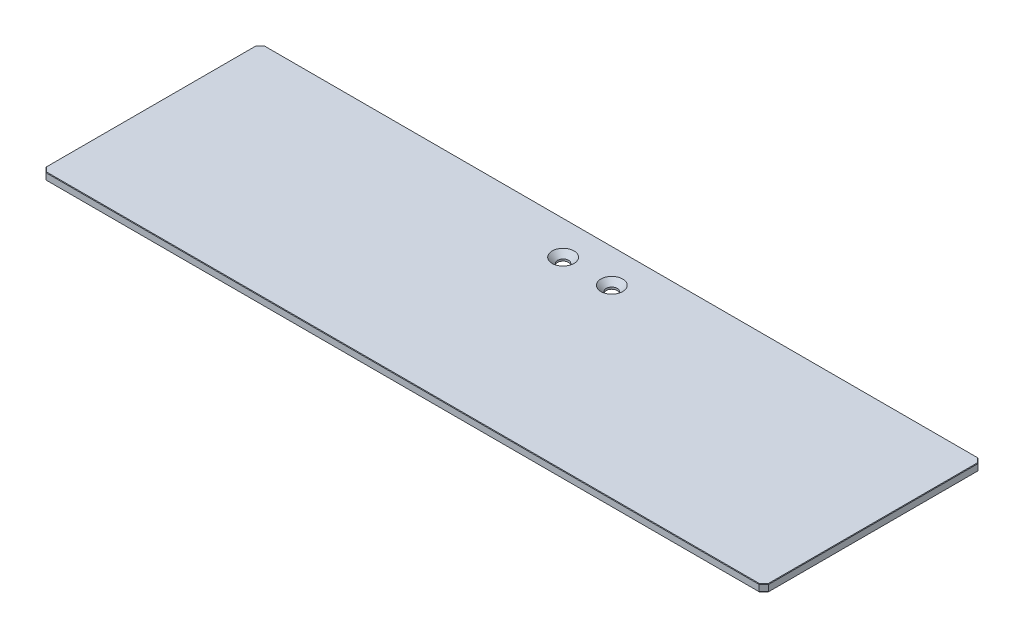
SolidWorks part; units mm, degrees
material "不锈钢"
ref_plane "Front" through (0, 0, 0) normal (0, 0, 1) x (1, 0, 0)
ref_plane "Top" through (0, 0, 0) normal (0, 1, 0) x (1, 0, 0)
ref_plane "Right" through (0, 0, 0) normal (1, 0, 0) x (0, 0, -1)
sketch "草图1" plane through (0, 0, 0) normal (0, 1, 0) x (1, 0, 0)
  line L1 (-148.5, 45) -> (148.5, 45)
  line L2 (-148.5, 45) -> (-148.5, -45)
  line L3 (-148.5, -45) -> (148.5, -45)
  line L4 (148.5, 45) -> (148.5, -45)
  line L5 (-148.5, 45) -> (148.5, -45) construction
  line L6 (-148.5, -45) -> (148.5, 45) construction
  point P0 (0, 0)
  dimension "D1" = 90
  dimension "D2" = 297
extrude "凸台-拉伸1" add sketch "草图1" along normal blind 3
hole_wizard "M4 六角凹锥坑螺钉的锥形沉头孔1" positions "草图3" profile "草图2" countersink size "M4" standard "Iso" end condition through all
sketch "草图3" plane through (0, 3, 0) normal (0, 1, 0) x (1, 0, 0)
  line L0 (0, 0) -> (0, -45) construction
  line L1 (-148.5, -45) -> (148.5, -45) construction
  line L3 (148.5, 45) -> (-148.5, 45) construction
  point P0 (-10, 31)
  point P2 (10, 31)
  dimension "D1" = 20
  dimension "D2" = 14
sketch "草图2" plane through (-10, 3, -31) normal (1, 0, 0) x (0, 0, 1)
  line L0 (0, 0) -> (0, 3)
  line L1 (0, 3) -> (2.25, 3)
  line L2 (2.25, 3) -> (2.25, 2.23)
  line L3 (2.25, 2.23) -> (4.48, 0)
  line L5 (4.48, 0) -> (0, 0)
  line L6 (-2.25, 2.23) -> (-4.48, 0) construction
  line L11 (0, -6.35) -> (0, 107.95) construction
  dimension "通孔孔直径" = 4.5
  dimension "通孔孔深度" = 3
  dimension "近端锥形沉头孔直径" = 8.96
  dimension "近端锥形沉头孔角度" = 90
chamfer "倒角1" distance 2 angle 45 4 edges at (148.5, 1.5, -45) (148.5, 1.5, 45) (-148.5, 1.5, 45) (-148.5, 1.5, -45)
chamfer "倒角2" distance 0.2 angle 45 8 edges at (-147.5, 0, 44) (0, 0, 45) (147.5, 0, 44) (148.5, 0, 0) (147.5, 0, -44) (0, 0, -45) (-147.5, 0, -44) (-148.5, 0, 0)
chamfer "倒角3" distance 0.2 angle 45 8 edges at (147.5, 3, -44) (148.5, 3, 0) (147.5, 3, 44) (0, 3, 45) (-147.5, 3, 44) (-148.5, 3, 0) (-147.5, 3, -44) (0, 3, -45)
